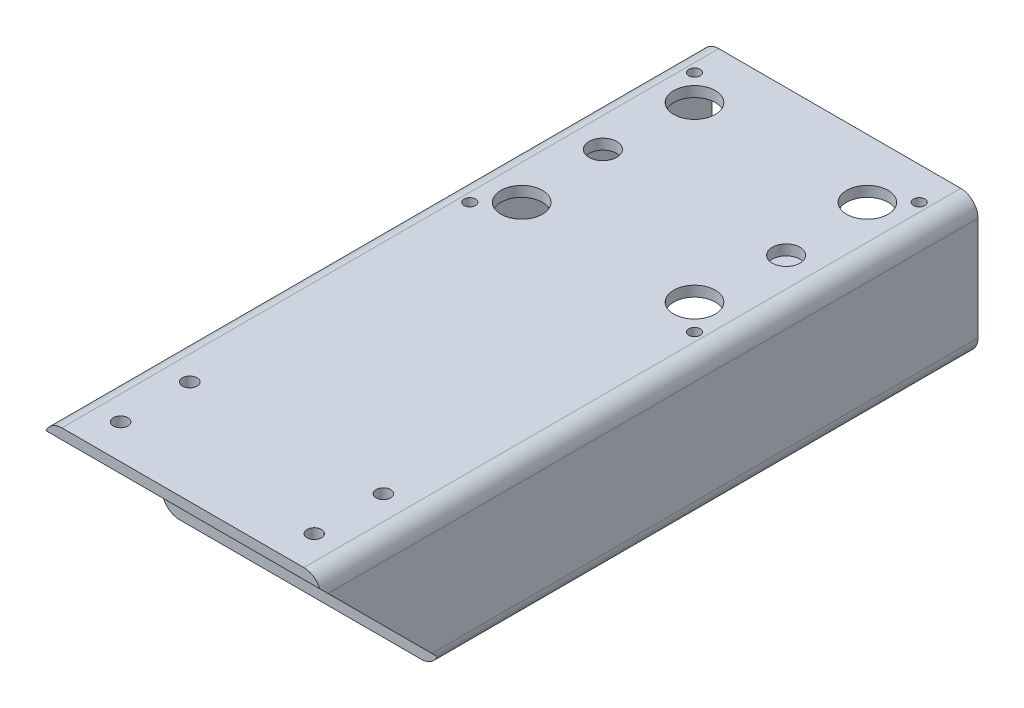
SolidWorks part; units mm, degrees
ref_plane "前视" through (0, 0, 0) normal (0, 0, 1) x (1, 0, 0)
ref_plane "上视" through (0, 0, 0) normal (0, 1, 0) x (1, 0, 0)
ref_plane "右视" through (0, 0, 0) normal (1, 0, 0) x (0, 0, -1)
sketch "草图1" plane through (0, 0, 0) normal (0, 0, 1) x (1, 0, 0)
  line L0 (-37, 15) -> (-37, -15)
  line L1 (-35, 20) -> (35, 20)
  line L2 (-40, 15) -> (-40, -15)
  line L3 (-35, -20) -> (35, -20)
  line L4 (40, 15) -> (40, -15)
  line L5 (-40, 20) -> (40, -20) construction
  line L6 (-40, -20) -> (40, 20) construction
  line L7 (-35, -17) -> (35, -17)
  line L8 (37, 15) -> (37, -15)
  line L9 (-35, 17) -> (35, 17)
  arc A0 (-40, -15) -> (-35, -20) centre (-35, -15) ccw
  arc A1 (35, -20) -> (40, -15) centre (35, -15) ccw
  arc A2 (40, 15) -> (35, 20) centre (35, 15) ccw
  arc A3 (-35, 20) -> (-40, 15) centre (-35, 15) ccw
  arc A4 (-37, -15) -> (-35, -17) centre (-35, -15) ccw
  arc A5 (35, -17) -> (37, -15) centre (35, -15) ccw
  arc A6 (37, 15) -> (35, 17) centre (35, 15) ccw
  arc A7 (-35, 17) -> (-37, 15) centre (-35, 15) ccw
  point P0 (0, 0)
  dimension "D3" = 5
  dimension "D1" = 80
  dimension "D2" = 40
  dimension "D4" = 3
extrude "凸台-拉伸1" add sketch "草图1" along normal blind 190
sketch "草图6" plane through (0, -20, 0) normal (0, -1, 0) x (1, 0, 0)
  line L0 (-35, 0) -> (35, 0) construction
  circle A0 centre (0, 42) radius 23.25
  dimension "D2" = 46.5
  dimension "D1" = 42
extrude "切除-拉伸1" cut sketch "草图6" against normal up to surface (3 mm away) up to face at (0, -17, 95)
hole_wizard "Ø6.5 (6.5) 直径孔1" positions "草图3" profile "草图2" hole size "Ø6.5" standard "Gb" end condition through all
sketch "草图3" plane through (0, 20, 0) normal (0, 1, 0) x (1, 0, 0)
  line L3 (0, -42) -> (0, -13.8326) construction
  line L5 (0, -42) -> (29.785, -42) construction
  point P0 (-25, -17)
  point P3 (25, -17)
  point P6 (25, -67)
  point P9 (-25, -67)
  dimension "D1" = 50
  dimension "D2" = 50
sketch "草图2" plane through (-25, 20, 17) normal (1, 0, 0) x (0, 0, 1)
  line L0 (0, 0) -> (0, 40)
  line L1 (0, 40) -> (3.25, 40)
  line L2 (3.25, 40) -> (3.25, 0)
  line L5 (3.25, 0) -> (0, 0)
  line L11 (0, -6.35) -> (0, 107.95) construction
  dimension "通孔孔直径" = 6.5
  dimension "通孔孔深度" = 40
hole_wizard "Ø12.0 (12) 直径孔1" positions "草图5" profile "草图4" hole size "Ø12.0" standard "Gb"
sketch "草图5" plane through (0, 20, 0) normal (0, 1, 0) x (1, 0, 0)
  point P0 (-25, -17)
  point P3 (25, -17)
  point P6 (25, -67)
  point P9 (-25, -67)
sketch "草图4" plane through (-25, 20, 17) normal (1, 0, 0) x (0, 0, 1)
  line L0 (0, 0) -> (0, 6.6042)
  line L1 (0, 6.6042) -> (6, 2.999)
  line L2 (6, 2.999) -> (6, 0)
  line L5 (6, 0) -> (0, 0)
  line L10 (0, 6.6042) -> (-6, 2.999) construction
  line L11 (0, -6.35) -> (0, 107.95) construction
  dimension "孔直径" = 12
  dimension "孔深度" = 2.999
  dimension "导头角度" = 118
hole_wizard "M4 螺纹孔1" positions "草图8" profile "草图7" tap size "M4" standard "Gb"
sketch "草图8" plane through (0, 20, 0) normal (0, 1, 0) x (1, 0, 0)
  line L0 (0, -42) -> (0, -10.966) construction
  line L2 (0, -42) -> (44.1531, -42) construction
  point P0 (-32.5, -9.5)
  point P2 (32.5, -9.5)
  point P4 (32.5, -74.5)
  point P6 (-32.5, -74.5)
  dimension "D1" = 65
  dimension "D2" = 65
sketch "草图7" plane through (-32.5, 20, 9.5) normal (1, 0, 0) x (0, 0, 1)
  line L0 (0, 0) -> (0, 3.9904)
  line L1 (0, 3.9904) -> (1.65, 2.999)
  line L2 (1.65, 2.999) -> (1.65, 0)
  line L5 (1.65, 0) -> (0, 0)
  line L10 (0, 3.9904) -> (-1.65, 2.999) construction
  line L11 (0, -6.35) -> (0, 107.95) construction
  dimension "螺纹孔钻头直径" = 3.3
  dimension "螺纹孔钻头深度" = 2.999
  dimension "导头角度" = 118
cosmetic thread "孔螺蚊线1" parameters "D1"=3, "D2"=4
cosmetic thread "孔螺蚊线2" parameters "D1"=3, "D2"=4
cosmetic thread "孔螺蚊线3" parameters "D1"=3, "D2"=4
cosmetic thread "孔螺蚊线4" parameters "D1"=3, "D2"=4
sketch "草图9" plane through (40, 0, 0) normal (1, 0, 0) x (0, 0, -1)
  line L0 (-190, 17) -> (-190, -20)
  line L1 (-190, -20) -> (-156, -20)
  line L2 (-156, -17) -> (-190, 17)
  line L3 (-190, -15) -> (-190, 15) construction
  line L4 (-190, -20) -> (0, -20) construction
  line L5 (-156, -20) -> (-156, -17)
  dimension "D1" = 45
  dimension "D2" = 3
extrude "切除-拉伸2" cut sketch "草图9" against normal through all
sketch "草图12" plane through (0, 17, 0) normal (0, -1, 0) x (1, 0, 0)
  line L0 (0, 0) -> (0, 225.4116) construction
  line L2 (35, 190) -> (-35, 190) construction
  circle A0 centre (-28, 160) radius 5
  circle A1 centre (-28, 180) radius 5
  circle A2 centre (28, 160) radius 5
  circle A3 centre (28, 180) radius 5
  dimension "D1" = 10
  dimension "D2" = 10
  dimension "D3" = 56
  dimension "D4" = 20
extrude "凸台-拉伸2" add sketch "草图12" along normal blind 3
hole_wizard "M5 螺纹孔1" positions "草图14" profile "草图13" tap size "M5" standard "Gb"
sketch "草图14" plane through (0, 20, 0) normal (0, 1, 0) x (1, 0, 0)
  point P0 (-28, -160)
  point P3 (-28, -180)
  point P6 (28, -160)
  point P9 (28, -180)
sketch "草图13" plane through (-28, 20, 160) normal (1, 0, 0) x (0, 0, 1)
  line L0 (0, 0) -> (0, 7.2608)
  line L1 (0, 7.2608) -> (2.1, 5.999)
  line L2 (2.1, 5.999) -> (2.1, 0)
  line L5 (2.1, 0) -> (0, 0)
  line L10 (0, 7.2608) -> (-2.1, 5.999) construction
  line L11 (0, -6.35) -> (0, 107.95) construction
  dimension "螺纹孔钻头直径" = 4.2
  dimension "螺纹孔钻头深度" = 5.999
  dimension "导头角度" = 118
cosmetic thread "孔螺蚊线8" parameters "D1"=6, "D2"=5
cosmetic thread "孔螺蚊线9" parameters "D1"=6, "D2"=5
cosmetic thread "孔螺蚊线10" parameters "D1"=6, "D2"=5
cosmetic thread "孔螺蚊线11" parameters "D1"=6, "D2"=5
hole_wizard "M3 螺纹孔1" positions "草图16" profile "草图15" tap size "M3" standard "Gb"
sketch "草图16" plane through (0, -20, 0) normal (0, -1, 0) x (-1, 0, 0)
  line L0 (0, -42) -> (46.5526, -42) construction
  line L2 (0, -42) -> (0, -50042) construction
  point P0 (26.5, -42)
  point P2 (-26.5, -42)
  dimension "D1" = 53
sketch "草图15" plane through (-26.5, -20, 42) normal (1, 0, 0) x (0, 0, -1)
  line L0 (0, 0) -> (0, 3)
  line L1 (0, 3) -> (1.25, 3)
  line L2 (1.25, 3) -> (1.25, 0)
  line L5 (1.25, 0) -> (0, 0)
  line L11 (0, -6.35) -> (0, 107.95) construction
  dimension "通孔螺纹孔钻头直径" = 2.5
  dimension "通孔螺纹孔钻头深度" = 3
cosmetic thread "孔螺蚊线12" parameters "D2"=3
cosmetic thread "孔螺蚊线13" parameters "D2"=3
sketch "草图17" plane through (0, 20, 0) normal (0, 1, 0) x (1, 0, 0)
  circle A0 centre (-26.5, -42) radius 4
  circle A1 centre (26.5, -42) radius 4
  dimension "D1" = 8
extrude "切除-拉伸3" cut sketch "草图17" against normal up to next
